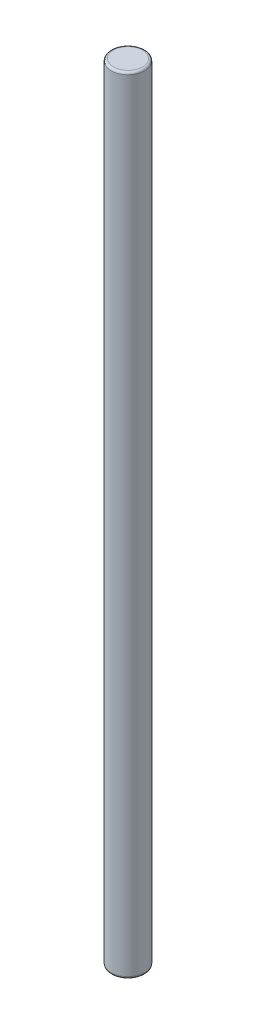
SolidWorks part; units mm, degrees
ref_plane "Front Plane" through (0, 0, 0) normal (0, 0, 1) x (1, 0, 0)
ref_plane "Top Plane" through (0, 0, 0) normal (0, 1, 0) x (1, 0, 0)
ref_plane "Right Plane" through (0, 0, 0) normal (1, 0, 0) x (0, 0, -1)
other "Configuration Table"
sketch "Sketch1" plane through (0, 0, 0) normal (0, 1, 0) x (1, 0, 0)
  circle A0 centre (0, 0) radius 1.5
  dimension "D1" = 3
extrude "Boss-Extrude1" add sketch "Sketch1" along normal blind 70
fillet "Fillet1" radius 0.2 2 edges at (0, 0, 1.5) (0, 70, 1.5)
